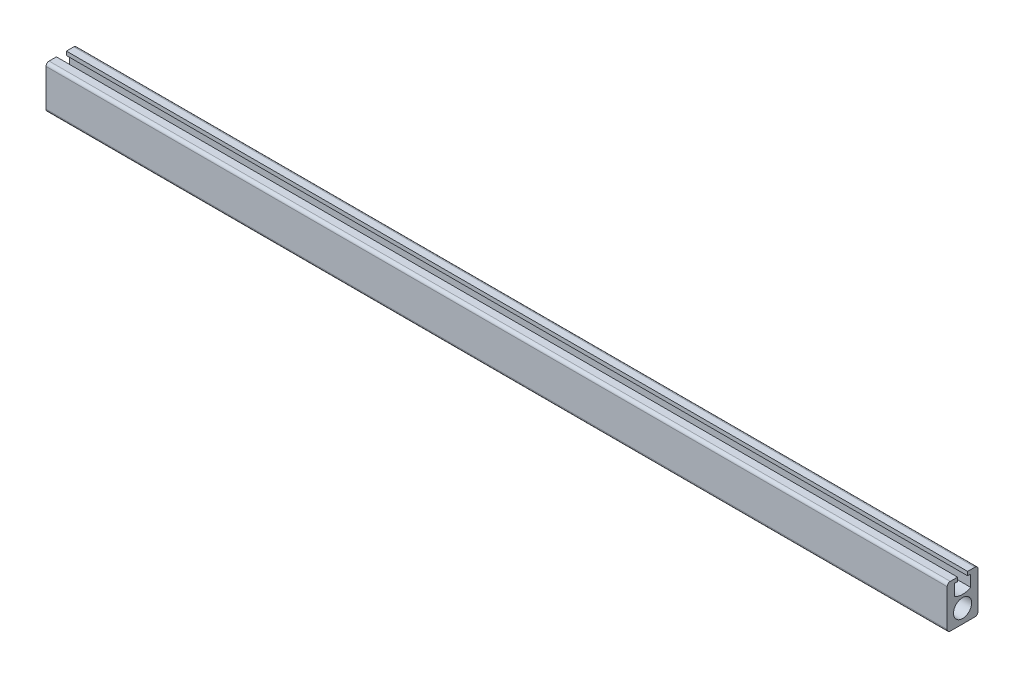
from build123d import *

# Parameters (mm, degrees)
SKETCH1_R               = 5.75
EXTRUDE1_DEPTH          = 585
FILLET1_R               = 2
G1_4_TAPPED_HOLE1_D     = 11.8
G1_4_TAPPED_HOLE1_DEPTH = 30.32
G1_4_TAPPED_HOLE1_TIP   = 3.545077652
G1_4_TAPPED_HOLE2_D     = 11.8
G1_4_TAPPED_HOLE2_DEPTH = 30.32
G1_4_TAPPED_HOLE2_TIP   = 3.545077652
M5_TAPPED_HOLE2_D       = 4.2
M5_TAPPED_HOLE2_DEPTH   = 8
M5_TAPPED_HOLE2_TIP     = 1.2618073
G1_4_TAPPED_HOLE7_D     = 11.8
G1_4_TAPPED_HOLE7_DEPTH = 10
G1_4_TAPPED_HOLE7_TIP   = 3.545077652


with BuildPart() as part:
    # Sketch1 → Extrude1 (new body)
    with BuildSketch(Plane(origin=(0, 0, 0), x_dir=(0, 0, -1), z_dir=(1, 0, 0))):
        with BuildLine():
            Line((-3.25, 19), (-3.25, 16.5))
            Line((-3.25, 16.5), (-5.25, 16.5))
            Line((-5.25, 16.5), (-5.25, 9))
            ThreePointArc((-5.25, 9), (0, 7.705643002), (5.25, 9))
            Line((5.25, 9), (5.25, 16.5))
            Line((5.25, 16.5), (3.25, 16.5))
            Line((3.25, 16.5), (3.25, 19))
            Line((3.25, 19), (10, 19))
            Line((10, 19), (10, -9))
            Line((10, -9), (-10, -9))
            Line((-10, -9), (-10, 19))
            Line((-10, 19), (-3.25, 19))
        make_face()
        Circle(SKETCH1_R, mode=Mode.SUBTRACT)
    extrude(amount=EXTRUDE1_DEPTH)

    # Fillet1
    fillet1_edges = [part.edges().sort_by_distance(p)[0] for p in [
        (292.5, 19, 10),
        (292.5, 19, -10),
        (292.5, -9, -10),
        (292.5, -9, 10),
    ]]
    fillet(fillet1_edges, radius=FILLET1_R)

    # G1/4 Tapped Hole1
    with Locations(Plane.ZY):
        with Locations((0, 0)):
            Hole(G1_4_TAPPED_HOLE1_D / 2, depth=G1_4_TAPPED_HOLE1_DEPTH)
            with Locations((0, 0, -(G1_4_TAPPED_HOLE1_DEPTH + G1_4_TAPPED_HOLE1_TIP / 2))):  # 118° drill point
                Cone(0, G1_4_TAPPED_HOLE1_D / 2, G1_4_TAPPED_HOLE1_TIP, mode=Mode.SUBTRACT)

    # G1/4 Tapped Hole2
    with Locations(Plane(origin=(585, 0, 0), x_dir=(0, 0, -1), z_dir=(1, 0, 0))):
        with Locations((0, 0)):
            Hole(G1_4_TAPPED_HOLE2_D / 2, depth=G1_4_TAPPED_HOLE2_DEPTH)
            with Locations((0, 0, -(G1_4_TAPPED_HOLE2_DEPTH + G1_4_TAPPED_HOLE2_TIP / 2))):  # 118° drill point
                Cone(0, G1_4_TAPPED_HOLE2_D / 2, G1_4_TAPPED_HOLE2_TIP, mode=Mode.SUBTRACT)

    # M5 Tapped Hole2
    with Locations(Plane(origin=(0, 0, -10), x_dir=(-1, 0, 0), z_dir=(0, 0, -1))):
        with Locations((-565, 0), (-495, 0), (-425, 0), (-355, 0), (-230, 0), (-160, 0), (-90, 0), (-20, 0)):
            Hole(M5_TAPPED_HOLE2_D / 2, depth=M5_TAPPED_HOLE2_DEPTH)
            with Locations((0, 0, -(M5_TAPPED_HOLE2_DEPTH + M5_TAPPED_HOLE2_TIP / 2))):  # 118° drill point
                Cone(0, M5_TAPPED_HOLE2_D / 2, M5_TAPPED_HOLE2_TIP, mode=Mode.SUBTRACT)

    # G1/4 Tapped Hole7
    with Locations(Plane(origin=(0, 0, -10), x_dir=(-1, 0, 0), z_dir=(0, 0, -1))):
        with Locations((-292.5, 0)):
            Hole(G1_4_TAPPED_HOLE7_D / 2, depth=G1_4_TAPPED_HOLE7_DEPTH)
            with Locations((0, 0, -(G1_4_TAPPED_HOLE7_DEPTH + G1_4_TAPPED_HOLE7_TIP / 2))):  # 118° drill point
                Cone(0, G1_4_TAPPED_HOLE7_D / 2, G1_4_TAPPED_HOLE7_TIP, mode=Mode.SUBTRACT)


solid = part.part
